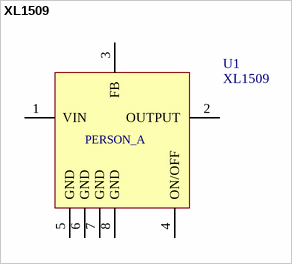
[diagram p0: symbol XL1509]
# Altium schematic symbol library MISC84315-3.SchLib: 1 symbol
Pins are listed as number, name and electrical type; pins without a type are passive.


## XL1509
designator U1
footprint ESOP8
pins: 1 VIN, 2 OUTPUT, 3 FB, 4 ON/OFF, 5 GND, 6 GND, 7 GND, 8 GND